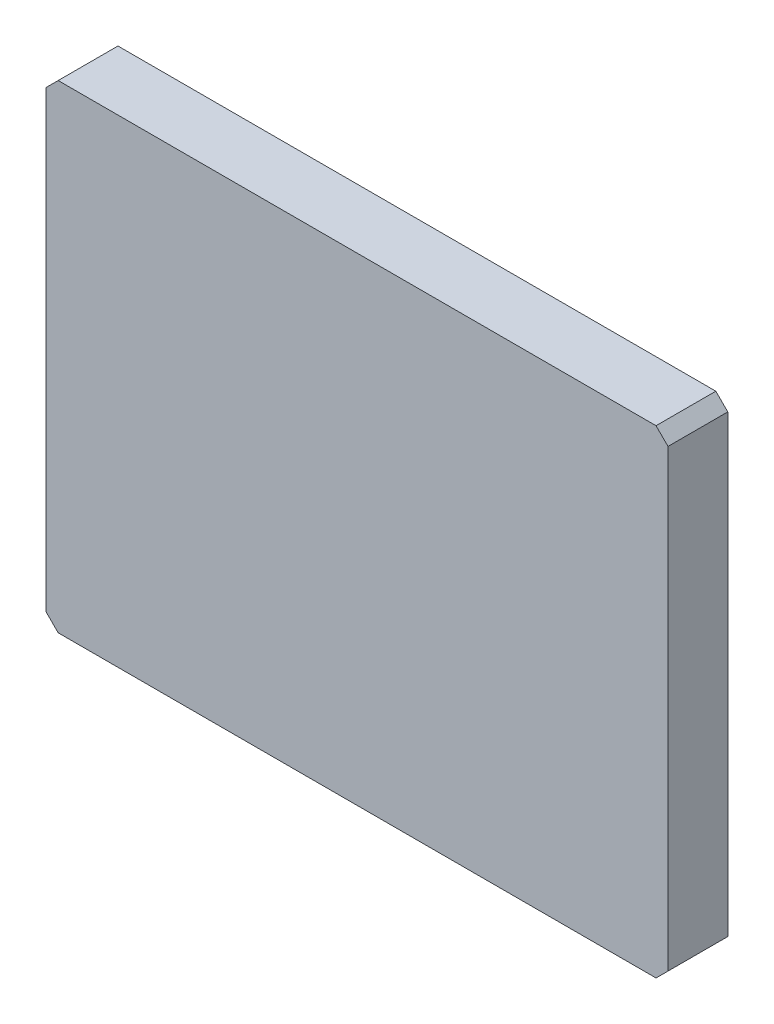
SolidWorks part; units mm, degrees
material "Q235-A "
ref_plane "前视基准面" through (0, 0, 0) normal (0, 0, 1) x (1, 0, 0)
ref_plane "上视基准面" through (0, 0, 0) normal (0, 1, 0) x (1, 0, 0)
ref_plane "右视基准面" through (0, 0, 0) normal (1, 0, 0) x (0, 0, -1)
sketch "草图1" plane through (0, 0, 0) normal (0, 0, 1) x (1, 0, 0)
  line L1 (-130, 100) -> (130, 100)
  line L2 (-130, 100) -> (-130, -100)
  line L3 (-130, -100) -> (130, -100)
  line L4 (130, 100) -> (130, -100)
  line L5 (-130, 100) -> (130, -100) construction
  line L6 (-130, -100) -> (130, 100) construction
  point P0 (0, 0)
  dimension "D1" = 260
  dimension "D2" = 200
extrude "凸台-拉伸1" add sketch "草图1" along normal blind 25
chamfer "倒角1" distance 5 angle 45 4 edges at (-130, -100, 12.5) (130, -100, 12.5) (-130, 100, 12.5) (130, 100, 12.5)
